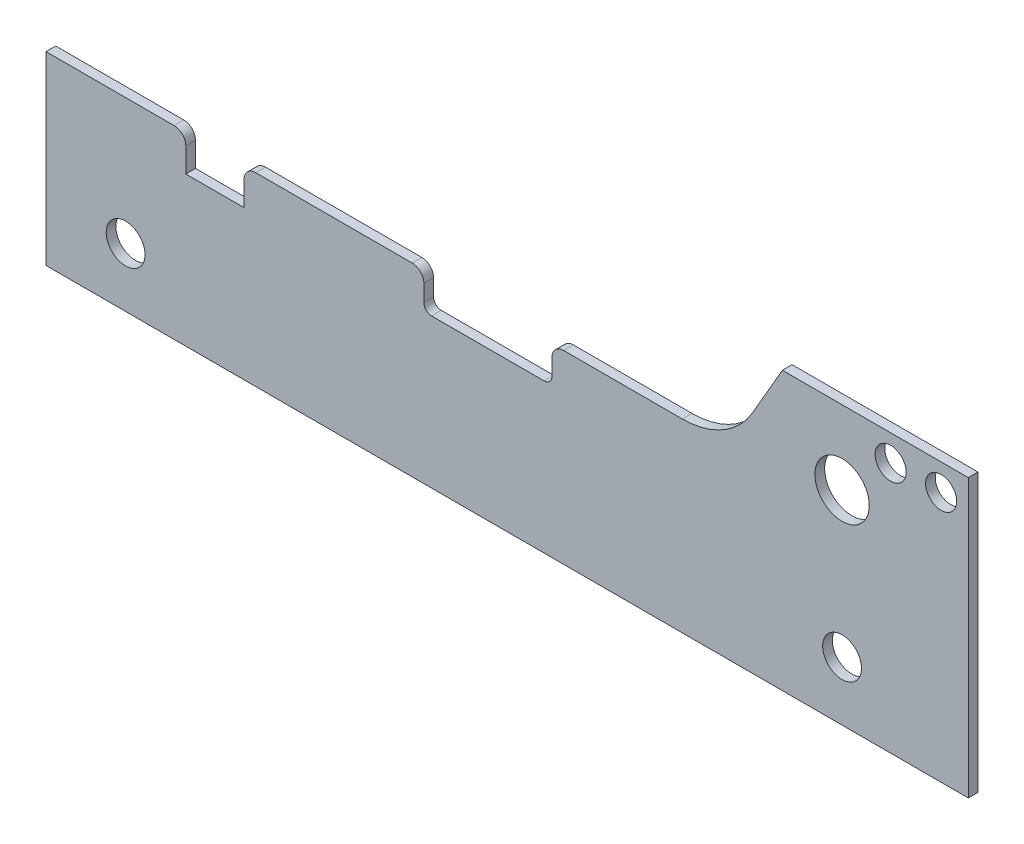
from build123d import *

# Parameters (mm, degrees)
SKETCH1_R           = 50
SKETCH1_R_2         = 70
SKETCH1_R_3         = 40
BOSS_EXTRUDE1_DEPTH = 25


with BuildPart() as part:
    # Sketch1 → Boss-Extrude1 (new body)
    with BuildSketch(Plane.XY):
        with BuildLine():
            Line((0, 0), (0, 477))
            Line((0, 477), (330, 477))
            ThreePointArc((330, 477), (351.213203436, 468.213203436), (360, 447))
            Line((360, 447), (360, 384))
            Line((360, 384), (510, 384))
            Line((510, 384), (510, 447))
            ThreePointArc((510, 447), (518.786796564, 468.213203436), (540, 477))
            Line((540, 477), (943, 477))
            ThreePointArc((943, 477), (964.213203436, 468.213203436), (973, 447))
            Line((973, 447), (973, 404))
            ThreePointArc((973, 404), (978.857864376, 389.857864376), (993, 384))
            Line((993, 384), (1283, 384))
            ThreePointArc((1283, 384), (1297.142135624, 389.857864376), (1303, 404))
            Line((1303, 404), (1303, 447))
            ThreePointArc((1303, 447), (1311.786796564, 468.213203436), (1333, 477))
            Line((1333, 477), (1638.413104807, 477))
            ThreePointArc((1638.413104807, 477), (1742.913104807, 505.000690609), (1819.412414198, 581.5))
            Line((1819.412414198, 581.5), (1896.2, 714.5))
            Line((1896.2, 714.5), (2375, 714.5))
            Line((2375, 714.5), (2375, 0))
            Line((2375, 0), (0, 0))
        make_face()
        with Locations((205, 151.5)):
            Circle(SKETCH1_R, mode=Mode.SUBTRACT)
        with Locations((2050, 151.5)):
            Circle(SKETCH1_R, mode=Mode.SUBTRACT)
        with Locations((2050, 524.5)):
            Circle(SKETCH1_R_2, mode=Mode.SUBTRACT)
        with Locations((2305, 646.5)):
            Circle(SKETCH1_R_3, mode=Mode.SUBTRACT)
        with Locations((2175, 646.5)):
            Circle(SKETCH1_R_3, mode=Mode.SUBTRACT)
    extrude(amount=BOSS_EXTRUDE1_DEPTH)


solid = part.part
